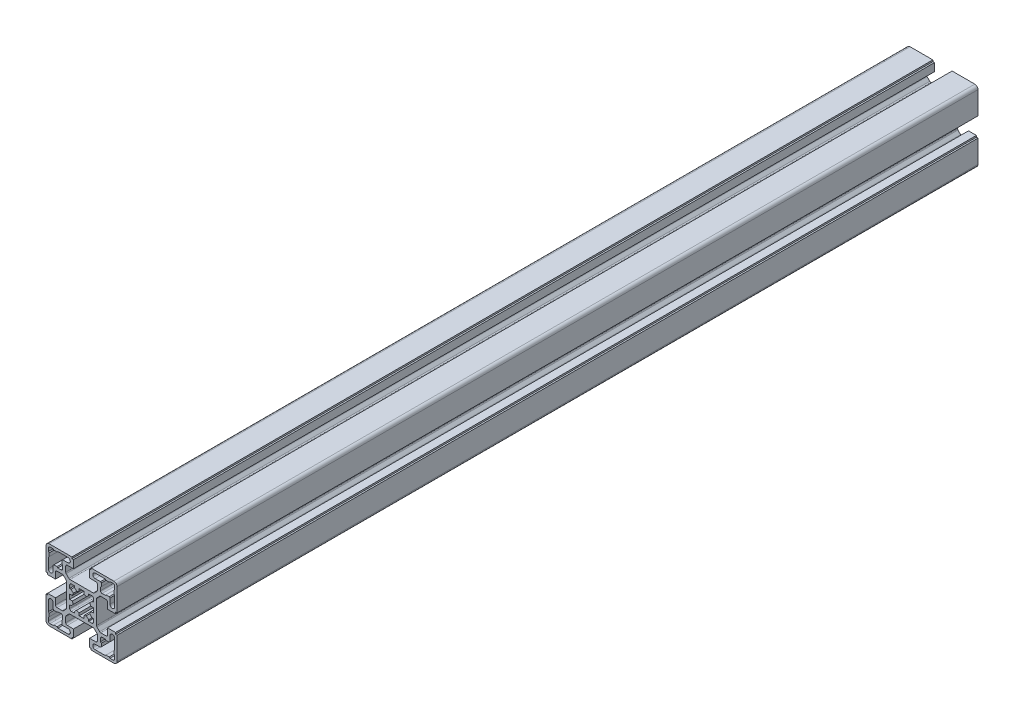
SolidWorks part; units mm, degrees
material "1.11.45.045045.04"
ref_plane "前视基准面" through (0, 0, 0) normal (0, 0, 1) x (1, 0, 0)
ref_plane "上视基准面" through (0, 0, 0) normal (0, 1, 0) x (1, 0, 0)
ref_plane "右视基准面" through (0, 0, 0) normal (1, 0, 0) x (0, 0, -1)
sketch "草图1" plane through (0, 0, 0) normal (0, 0, 1) x (1, 0, 0)
  line L0 (30.535, 44.0271) -> (29.0823, 45.4798)
  line L1 (31.4137, 44.0271) -> (30.535, 44.0271)
  line L2 (31.4137, 42.0271) -> (31.4137, 44.0271)
  line L3 (28.4137, 41.0271) -> (30.4137, 41.0271)
  line L4 (28.4137, 41.9058) -> (28.4137, 41.0271)
  line L5 (26.961, 43.3585) -> (28.4137, 41.9058)
  line L6 (25.4137, 41.0271) -> (25.4137, 42.7176)
  line L7 (22.4137, 41.0271) -> (25.4137, 41.0271)
  line L8 (22.4137, 42.7176) -> (22.4137, 41.0271)
  line L9 (19.4137, 41.9058) -> (20.8664, 43.3585)
  line L10 (19.4137, 41.0271) -> (19.4137, 41.9058)
  line L11 (17.4137, 41.0271) -> (19.4137, 41.0271)
  line L12 (16.4137, 44.0271) -> (16.4137, 42.0271)
  line L13 (17.2924, 44.0271) -> (16.4137, 44.0271)
  line L14 (18.7451, 45.4798) -> (17.2924, 44.0271)
  line L15 (16.4137, 47.0271) -> (18.1042, 47.0271)
  line L16 (16.4137, 50.0271) -> (16.4137, 47.0271)
  line L17 (18.1042, 50.0271) -> (16.4137, 50.0271)
  line L18 (17.2924, 53.0271) -> (18.7451, 51.5744)
  line L19 (16.4137, 53.0271) -> (17.2924, 53.0271)
  line L20 (16.4137, 55.0271) -> (16.4137, 53.0271)
  line L21 (19.4137, 56.0271) -> (17.4137, 56.0271)
  line L22 (19.4137, 55.1484) -> (19.4137, 56.0271)
  line L23 (20.8664, 53.6957) -> (19.4137, 55.1484)
  line L24 (22.4137, 56.0271) -> (22.4137, 54.3366)
  line L25 (25.4137, 56.0271) -> (22.4137, 56.0271)
  line L26 (25.4137, 54.3366) -> (25.4137, 56.0271)
  line L27 (28.4137, 55.1484) -> (26.961, 53.6957)
  line L28 (28.4137, 56.0271) -> (28.4137, 55.1484)
  line L29 (30.4137, 56.0271) -> (28.4137, 56.0271)
  line L30 (31.4137, 53.0271) -> (31.4137, 55.0271)
  line L31 (30.535, 53.0271) -> (31.4137, 53.0271)
  line L32 (29.0823, 51.5744) -> (30.535, 53.0271)
  line L33 (31.4137, 50.0271) -> (29.7232, 50.0271)
  line L34 (31.4137, 47.0271) -> (31.4137, 50.0271)
  line L35 (29.7232, 47.0271) -> (31.4137, 47.0271)
  line L36 (11.4137, 66.0271) -> (11.9137, 66.5271)
  line L37 (11.4137, 64.0271) -> (11.4137, 66.0271)
  line L38 (11.9137, 63.5271) -> (11.4137, 64.0271)
  line L39 (11.9137, 61.5271) -> (11.9137, 63.5271)
  line L40 (8.9137, 60.5271) -> (10.9137, 60.5271)
  line L41 (8.4137, 61.0271) -> (8.9137, 60.5271)
  line L42 (6.4137, 61.0271) -> (8.4137, 61.0271)
  line L43 (5.9137, 60.5271) -> (6.4137, 61.0271)
  line L44 (5.9137, 57.1271) -> (5.9137, 60.5271)
  line L45 (2.9137, 63.5271) -> (2.9137, 57.1271)
  line L46 (3.4137, 64.0271) -> (2.9137, 63.5271)
  line L47 (3.4137, 66.0271) -> (3.4137, 64.0271)
  line L48 (2.9137, 66.5271) -> (3.4137, 66.0271)
  line L49 (2.9137, 68.5271) -> (2.9137, 66.5271)
  line L50 (5.9137, 69.5271) -> (3.9137, 69.5271)
  line L51 (6.4137, 69.0271) -> (5.9137, 69.5271)
  line L52 (8.4137, 69.0271) -> (6.4137, 69.0271)
  line L53 (8.9137, 69.5271) -> (8.4137, 69.0271)
  line L54 (15.3137, 69.5271) -> (8.9137, 69.5271)
  line L55 (11.9137, 66.5271) -> (15.3137, 66.5271)
  line L56 (11.9137, 30.5271) -> (11.4137, 31.0271)
  line L57 (15.3137, 30.5271) -> (11.9137, 30.5271)
  line L58 (8.9137, 27.5271) -> (15.3137, 27.5271)
  line L59 (8.4137, 28.0271) -> (8.9137, 27.5271)
  line L60 (6.4137, 28.0271) -> (8.4137, 28.0271)
  line L61 (5.9137, 27.5271) -> (6.4137, 28.0271)
  line L62 (3.9137, 27.5271) -> (5.9137, 27.5271)
  line L63 (2.9137, 30.5271) -> (2.9137, 28.5271)
  line L64 (3.4137, 31.0271) -> (2.9137, 30.5271)
  line L65 (3.4137, 33.0271) -> (3.4137, 31.0271)
  line L66 (2.9137, 33.5271) -> (3.4137, 33.0271)
  line L67 (2.9137, 39.9271) -> (2.9137, 33.5271)
  line L68 (5.9137, 36.5271) -> (5.9137, 39.9271)
  line L69 (6.4137, 36.0271) -> (5.9137, 36.5271)
  line L70 (8.4137, 36.0271) -> (6.4137, 36.0271)
  line L71 (8.9137, 36.5271) -> (8.4137, 36.0271)
  line L72 (10.9137, 36.5271) -> (8.9137, 36.5271)
  line L73 (11.9137, 33.5271) -> (11.9137, 35.5271)
  line L74 (11.4137, 33.0271) -> (11.9137, 33.5271)
  line L75 (11.4137, 31.0271) -> (11.4137, 33.0271)
  line L76 (41.9137, 36.5271) -> (41.4137, 36.0271)
  line L77 (41.9137, 39.9271) -> (41.9137, 36.5271)
  line L78 (44.9137, 33.5271) -> (44.9137, 39.9271)
  line L79 (44.4137, 33.0271) -> (44.9137, 33.5271)
  line L80 (44.4137, 31.0271) -> (44.4137, 33.0271)
  line L81 (44.9137, 30.5271) -> (44.4137, 31.0271)
  line L82 (44.9137, 28.5271) -> (44.9137, 30.5271)
  line L83 (41.9137, 27.5271) -> (43.9137, 27.5271)
  line L84 (41.4137, 28.0271) -> (41.9137, 27.5271)
  line L85 (39.4137, 28.0271) -> (41.4137, 28.0271)
  line L86 (38.9137, 27.5271) -> (39.4137, 28.0271)
  line L87 (32.5137, 27.5271) -> (38.9137, 27.5271)
  line L88 (35.9137, 30.5271) -> (32.5137, 30.5271)
  line L89 (36.4137, 31.0271) -> (35.9137, 30.5271)
  line L90 (36.4137, 33.0271) -> (36.4137, 31.0271)
  line L91 (35.9137, 33.5271) -> (36.4137, 33.0271)
  line L92 (35.9137, 35.5271) -> (35.9137, 33.5271)
  line L93 (38.9137, 36.5271) -> (36.9137, 36.5271)
  line L94 (39.4137, 36.0271) -> (38.9137, 36.5271)
  line L95 (41.4137, 36.0271) -> (39.4137, 36.0271)
  line L96 (35.9137, 66.5271) -> (36.4137, 66.0271)
  line L97 (32.5137, 66.5271) -> (35.9137, 66.5271)
  line L98 (38.9137, 69.5271) -> (32.5137, 69.5271)
  line L99 (39.4137, 69.0271) -> (38.9137, 69.5271)
  line L100 (41.4137, 69.0271) -> (39.4137, 69.0271)
  line L101 (41.9137, 69.5271) -> (41.4137, 69.0271)
  line L102 (43.9137, 69.5271) -> (41.9137, 69.5271)
  line L103 (44.9137, 66.5271) -> (44.9137, 68.5271)
  line L104 (44.4137, 66.0271) -> (44.9137, 66.5271)
  line L105 (44.4137, 64.0271) -> (44.4137, 66.0271)
  line L106 (44.9137, 63.5271) -> (44.4137, 64.0271)
  line L107 (44.9137, 57.1271) -> (44.9137, 63.5271)
  line L108 (41.9137, 60.5271) -> (41.9137, 57.1271)
  line L109 (41.4137, 61.0271) -> (41.9137, 60.5271)
  line L110 (39.4137, 61.0271) -> (41.4137, 61.0271)
  line L111 (38.9137, 60.5271) -> (39.4137, 61.0271)
  line L112 (36.9137, 60.5271) -> (38.9137, 60.5271)
  line L113 (35.9137, 63.5271) -> (35.9137, 61.5271)
  line L114 (36.4137, 64.0271) -> (35.9137, 63.5271)
  line L115 (36.4137, 66.0271) -> (36.4137, 64.0271)
  line L116 (33.7066, 40.502) -> (35.3886, 38.82)
  line L117 (33.4137, 55.8451) -> (33.4137, 41.2091)
  line L118 (35.3886, 58.2342) -> (33.7066, 56.5522)
  line L119 (39.4137, 58.5271) -> (36.0957, 58.5271)
  line L120 (40.4137, 53.6271) -> (40.4137, 57.5271)
  line L121 (45.4137, 53.6271) -> (40.4137, 53.6271)
  line L122 (45.4137, 54.6271) -> (45.4137, 53.6271)
  line L123 (46.4137, 54.6271) -> (45.4137, 54.6271)
  line L124 (46.4137, 69.0271) -> (46.4137, 54.6271)
  line L125 (30.0137, 71.0271) -> (44.4137, 71.0271)
  line L126 (30.0137, 70.0271) -> (30.0137, 71.0271)
  line L127 (29.0137, 70.0271) -> (30.0137, 70.0271)
  line L128 (29.0137, 65.0271) -> (29.0137, 70.0271)
  line L129 (32.9137, 65.0271) -> (29.0137, 65.0271)
  line L130 (33.9137, 60.7091) -> (33.9137, 64.0271)
  line L131 (31.9388, 58.32) -> (33.6208, 60.002)
  line L132 (16.5957, 58.0271) -> (31.2317, 58.0271)
  line L133 (14.2066, 60.002) -> (15.8886, 58.32)
  line L134 (13.9137, 64.0271) -> (13.9137, 60.7091)
  line L135 (18.8137, 65.0271) -> (14.9137, 65.0271)
  line L136 (18.8137, 70.0271) -> (18.8137, 65.0271)
  line L137 (17.8137, 70.0271) -> (18.8137, 70.0271)
  line L138 (17.8137, 71.0271) -> (17.8137, 70.0271)
  line L139 (3.4137, 71.0271) -> (17.8137, 71.0271)
  line L140 (1.4137, 54.6271) -> (1.4137, 69.0271)
  line L141 (2.4137, 54.6271) -> (1.4137, 54.6271)
  line L142 (2.4137, 53.6271) -> (2.4137, 54.6271)
  line L143 (7.4137, 53.6271) -> (2.4137, 53.6271)
  line L144 (7.4137, 57.5271) -> (7.4137, 53.6271)
  line L145 (11.7317, 58.5271) -> (8.4137, 58.5271)
  line L146 (14.1208, 56.5522) -> (12.4388, 58.2342)
  line L147 (14.4137, 41.2091) -> (14.4137, 55.8451)
  line L148 (12.4388, 38.82) -> (14.1208, 40.502)
  line L149 (8.4137, 38.5271) -> (11.7317, 38.5271)
  line L150 (7.4137, 43.4271) -> (7.4137, 39.5271)
  line L151 (2.4137, 43.4271) -> (7.4137, 43.4271)
  line L152 (2.4137, 42.4271) -> (2.4137, 43.4271)
  line L153 (1.4137, 42.4271) -> (2.4137, 42.4271)
  line L154 (1.4137, 28.0271) -> (1.4137, 42.4271)
  line L155 (17.8137, 26.0271) -> (3.4137, 26.0271)
  line L156 (17.8137, 27.0271) -> (17.8137, 26.0271)
  line L157 (18.8137, 27.0271) -> (17.8137, 27.0271)
  line L158 (18.8137, 32.0271) -> (18.8137, 27.0271)
  line L159 (14.9137, 32.0271) -> (18.8137, 32.0271)
  line L160 (13.9137, 36.3451) -> (13.9137, 33.0271)
  line L161 (15.8886, 38.7342) -> (14.2066, 37.0522)
  line L162 (31.2317, 39.0271) -> (16.5957, 39.0271)
  line L163 (33.6208, 37.0522) -> (31.9388, 38.7342)
  line L164 (33.9137, 33.0271) -> (33.9137, 36.3451)
  line L165 (29.0137, 32.0271) -> (32.9137, 32.0271)
  line L166 (29.0137, 27.0271) -> (29.0137, 32.0271)
  line L167 (30.0137, 27.0271) -> (29.0137, 27.0271)
  line L168 (30.0137, 26.0271) -> (30.0137, 27.0271)
  line L169 (44.4137, 26.0271) -> (30.0137, 26.0271)
  line L170 (46.4137, 42.4271) -> (46.4137, 28.0271)
  line L171 (45.4137, 42.4271) -> (46.4137, 42.4271)
  line L172 (45.4137, 43.4271) -> (45.4137, 42.4271)
  line L173 (40.4137, 43.4271) -> (45.4137, 43.4271)
  line L174 (40.4137, 39.5271) -> (40.4137, 43.4271)
  line L175 (36.0957, 38.5271) -> (39.4137, 38.5271)
  arc A0 (30.4137, 41.0271) -> (31.4137, 42.0271) centre (30.4137, 42.0271) ccw
  arc A1 (25.4137, 42.7176) -> (26.961, 43.3585) centre (23.9137, 48.5271) ccw
  arc A2 (20.8664, 43.3585) -> (22.4137, 42.7176) centre (23.9137, 48.5271) ccw
  arc A3 (16.4137, 42.0271) -> (17.4137, 41.0271) centre (17.4137, 42.0271) ccw
  arc A4 (18.1042, 47.0271) -> (18.7451, 45.4798) centre (23.9137, 48.5271) ccw
  arc A5 (18.7451, 51.5744) -> (18.1042, 50.0271) centre (23.9137, 48.5271) ccw
  arc A6 (17.4137, 56.0271) -> (16.4137, 55.0271) centre (17.4137, 55.0271) ccw
  arc A7 (22.4137, 54.3366) -> (20.8664, 53.6957) centre (23.9137, 48.5271) ccw
  arc A8 (26.961, 53.6957) -> (25.4137, 54.3366) centre (23.9137, 48.5271) ccw
  arc A9 (31.4137, 55.0271) -> (30.4137, 56.0271) centre (30.4137, 55.0271) ccw
  arc A10 (29.7232, 50.0271) -> (29.0823, 51.5744) centre (23.9137, 48.5271) ccw
  arc A11 (29.0823, 45.4798) -> (29.7232, 47.0271) centre (23.9137, 48.5271) ccw
  arc A12 (10.9137, 60.5271) -> (11.9137, 61.5271) centre (10.9137, 61.5271) ccw
  arc A13 (2.9137, 57.1271) -> (5.9137, 57.1271) centre (4.4137, 57.1271) ccw
  arc A14 (3.9137, 69.5271) -> (2.9137, 68.5271) centre (3.9137, 68.5271) ccw
  arc A15 (15.3137, 66.5271) -> (15.3137, 69.5271) centre (15.3137, 68.0271) ccw
  arc A16 (15.3137, 27.5271) -> (15.3137, 30.5271) centre (15.3137, 29.0271) ccw
  arc A17 (2.9137, 28.5271) -> (3.9137, 27.5271) centre (3.9137, 28.5271) ccw
  arc A18 (5.9137, 39.9271) -> (2.9137, 39.9271) centre (4.4137, 39.9271) ccw
  arc A19 (11.9137, 35.5271) -> (10.9137, 36.5271) centre (10.9137, 35.5271) ccw
  arc A20 (44.9137, 39.9271) -> (41.9137, 39.9271) centre (43.4137, 39.9271) ccw
  arc A21 (43.9137, 27.5271) -> (44.9137, 28.5271) centre (43.9137, 28.5271) ccw
  arc A22 (32.5137, 30.5271) -> (32.5137, 27.5271) centre (32.5137, 29.0271) ccw
  arc A23 (36.9137, 36.5271) -> (35.9137, 35.5271) centre (36.9137, 35.5271) ccw
  arc A24 (32.5137, 69.5271) -> (32.5137, 66.5271) centre (32.5137, 68.0271) ccw
  arc A25 (44.9137, 68.5271) -> (43.9137, 69.5271) centre (43.9137, 68.5271) ccw
  arc A26 (41.9137, 57.1271) -> (44.9137, 57.1271) centre (43.4137, 57.1271) ccw
  arc A27 (35.9137, 61.5271) -> (36.9137, 60.5271) centre (36.9137, 61.5271) ccw
  arc A28 (35.3886, 38.82) -> (36.0957, 38.5271) centre (36.0957, 39.5271) ccw
  arc A29 (33.4137, 41.2091) -> (33.7066, 40.502) centre (34.4137, 41.2091) ccw
  arc A30 (33.7066, 56.5522) -> (33.4137, 55.8451) centre (34.4137, 55.8451) ccw
  arc A31 (36.0957, 58.5271) -> (35.3886, 58.2342) centre (36.0957, 57.5271) ccw
  arc A32 (40.4137, 57.5271) -> (39.4137, 58.5271) centre (39.4137, 57.5271) ccw
  arc A33 (46.4137, 69.0271) -> (44.4137, 71.0271) centre (44.4137, 69.0271) ccw
  arc A34 (33.9137, 64.0271) -> (32.9137, 65.0271) centre (32.9137, 64.0271) ccw
  arc A35 (33.6208, 60.002) -> (33.9137, 60.7091) centre (32.9137, 60.7091) ccw
  arc A36 (31.2317, 58.0271) -> (31.9388, 58.32) centre (31.2317, 59.0271) ccw
  arc A37 (15.8886, 58.32) -> (16.5957, 58.0271) centre (16.5957, 59.0271) ccw
  arc A38 (13.9137, 60.7091) -> (14.2066, 60.002) centre (14.9137, 60.7091) ccw
  arc A39 (14.9137, 65.0271) -> (13.9137, 64.0271) centre (14.9137, 64.0271) ccw
  arc A40 (3.4137, 71.0271) -> (1.4137, 69.0271) centre (3.4137, 69.0271) ccw
  arc A41 (8.4137, 58.5271) -> (7.4137, 57.5271) centre (8.4137, 57.5271) ccw
  arc A42 (12.4388, 58.2342) -> (11.7317, 58.5271) centre (11.7317, 57.5271) ccw
  arc A43 (14.4137, 55.8451) -> (14.1208, 56.5522) centre (13.4137, 55.8451) ccw
  arc A44 (14.1208, 40.502) -> (14.4137, 41.2091) centre (13.4137, 41.2091) ccw
  arc A45 (11.7317, 38.5271) -> (12.4388, 38.82) centre (11.7317, 39.5271) ccw
  arc A46 (7.4137, 39.5271) -> (8.4137, 38.5271) centre (8.4137, 39.5271) ccw
  arc A47 (1.4137, 28.0271) -> (3.4137, 26.0271) centre (3.4137, 28.0271) ccw
  arc A48 (13.9137, 33.0271) -> (14.9137, 32.0271) centre (14.9137, 33.0271) ccw
  arc A49 (14.2066, 37.0522) -> (13.9137, 36.3451) centre (14.9137, 36.3451) ccw
  arc A50 (16.5957, 39.0271) -> (15.8886, 38.7342) centre (16.5957, 38.0271) ccw
  arc A51 (31.9388, 38.7342) -> (31.2317, 39.0271) centre (31.2317, 38.0271) ccw
  arc A52 (33.9137, 36.3451) -> (33.6208, 37.0522) centre (32.9137, 36.3451) ccw
  arc A53 (32.9137, 32.0271) -> (33.9137, 33.0271) centre (32.9137, 33.0271) ccw
  arc A54 (44.4137, 26.0271) -> (46.4137, 28.0271) centre (44.4137, 28.0271) ccw
  arc A55 (39.4137, 38.5271) -> (40.4137, 39.5271) centre (39.4137, 39.5271) ccw
extrude "拉伸1" add sketch "草图1" along normal blind 545
